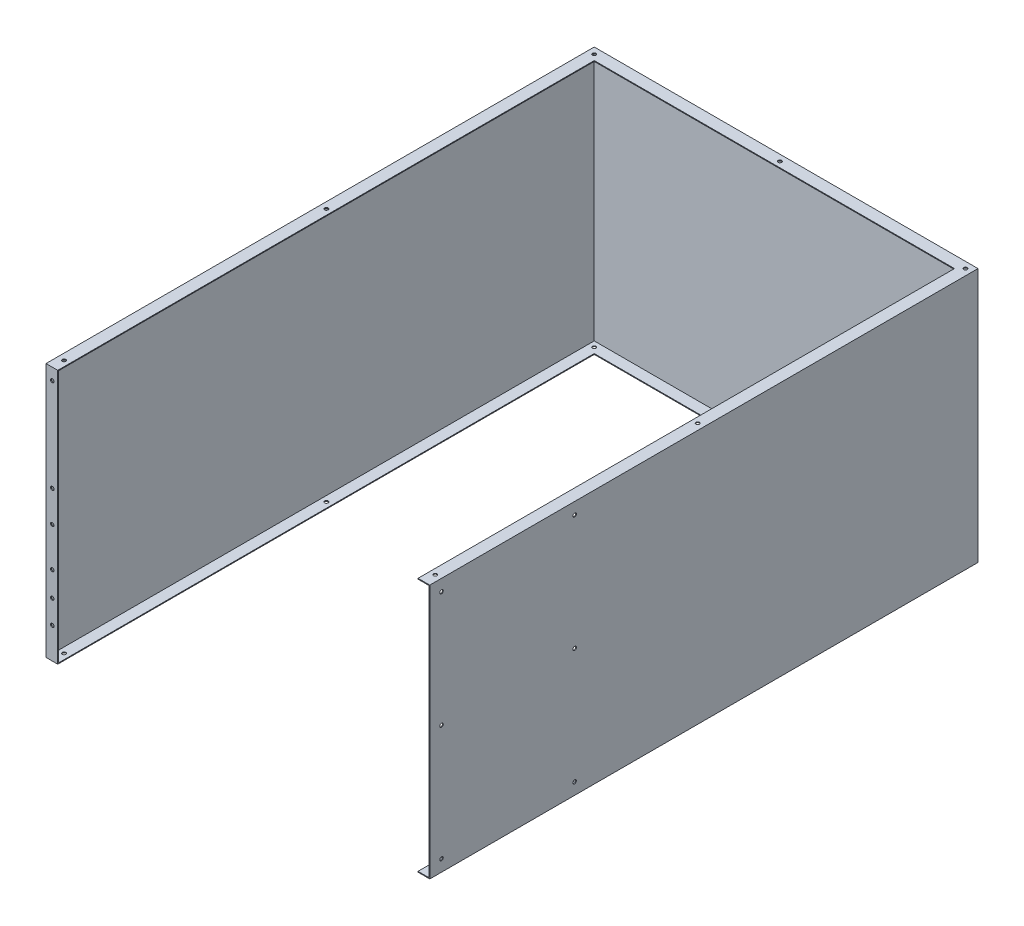
SolidWorks part; units mm, degrees
ref_plane "前视" through (0, 0, 0) normal (0, 0, 1) x (1, 0, 0)
ref_plane "上视" through (0, 0, 0) normal (0, 1, 0) x (1, 0, 0)
ref_plane "右视" through (0, 0, 0) normal (1, 0, 0) x (0, 0, -1)
sketch "草图1" plane through (0, 0, 0) normal (0, 1, 0) x (1, 0, 0)
  line L0 (0, 0) -> (0, 59.963) construction
  line L1 (0, 0) -> (65.7983, 0) construction
  line L2 (-490, 700) -> (490, 700)
  line L3 (490, 700) -> (490, -700)
  line L4 (-490, 700) -> (-490, -700)
  line L5 (-490, -700) -> (-488, -700)
  line L6 (-488, -700) -> (-488, 698)
  line L7 (490, -700) -> (488, -700)
  line L8 (488, -700) -> (488, 698)
  line L9 (488, 698) -> (-488, 698)
  dimension "D1" = 700
  dimension "D2" = 980
  dimension "D3" = 1400
  dimension "D4" = 490
  dimension "D5" = 1398
extrude "凸台-拉伸1" add sketch "草图1" along normal mid plane 650
sketch "草图2" plane through (0, 325, 0) normal (0, 1, 0) x (1, 0, 0)
  line L0 (-490, 700) -> (-490, -700)
  line L1 (-490, -700) -> (-460, -700)
  line L2 (-490, 700) -> (490, 700)
  line L3 (490, 700) -> (490, -700)
  line L4 (490, -700) -> (460, -700)
  line L5 (460, -700) -> (460, 670)
  line L6 (-460, -700) -> (-460, 670)
  line L7 (-460, 670) -> (460, 670)
  dimension "D1" = 30
  dimension "D2" = 30
  dimension "D3" = 30
extrude "凸台-拉伸2" add sketch "草图2" against normal blind 2
sketch "草图3" plane through (0, -325, 0) normal (0, -1, 0) x (1, 0, 0)
  line L0 (490, -700) -> (490, 700)
  line L1 (490, 700) -> (460, 700)
  line L2 (460, 700) -> (460, -670)
  line L3 (460, -670) -> (-460, -670)
  line L4 (-460, 700) -> (-460, -670) construction
  line L5 (-460, -670) -> (460, -670) construction
  line L6 (-460, -670) -> (-460, 700)
  line L7 (-460, 700) -> (-490, 700)
  line L8 (-490, 700) -> (-490, -700)
  line L9 (-490, -700) -> (490, -700)
extrude "凸台-拉伸3" add sketch "草图3" against normal blind 2
sketch "草图5" plane through (0, 0, 700) normal (0, 0, 1) x (1, 0, 0)
  line L0 (-490, 325) -> (-490, -325)
  line L1 (-490, -325) -> (-460, -325)
  line L2 (-460, -325) -> (-460, 325)
  line L3 (-460, 325) -> (-490, 325)
extrude "凸台-拉伸4" add sketch "草图5" against normal blind 2
ref_plane "基准面1" through (0, 150, 0) normal (0, 1, 0) x (-1, 0, 0)
sketch "草图6" plane through (0, 0, 698) normal (0, 0, -1) x (-1, 0, 0)
  line L0 (474, -323) -> (474, 491.326) construction
  line L1 (460, -323) -> (488, -323) construction
  line L2 (490, -325) -> (460, -325) construction
  line L3 (490, 325) -> (460, 325) construction
  circle A0 centre (474, -246) radius 4.5
  circle A1 centre (474, -186) radius 4.5
  circle A2 centre (474, 295) radius 4.5
  circle A3 centre (474, 57) radius 4.5
  circle A4 centre (474, -23) radius 4.5
  circle A5 centre (474, -123) radius 4.5
  dimension "D1" = 9
  dimension "D2" = 79
  dimension "D3" = 9
  dimension "D4" = 60
  dimension "D5" = 9
  dimension "D6" = 9
  dimension "D7" = 30
  dimension "D8" = 238
  dimension "D9" = 9
  dimension "D10" = 9
  dimension "D11" = 100
  dimension "D12" = 80
extrude "切除-拉伸1" cut sketch "草图6" against normal blind 10
sketch "草图7" plane through (0, 323, 0) normal (0, -1, 0) x (1, 0, 0)
  line L0 (-490, 0) -> (665.5888, 0) construction
  line L1 (-490, -700) -> (-490, 700) construction
  line L6 (-490, 700) -> (-460, 700) construction
  line L8 (0, -684) -> (0, -30.3843) construction
  line L9 (474, 700) -> (474, -684)
  line L10 (474, -684) -> (-474, -684)
  line L11 (-474, -684) -> (-474, 700)
  line L12 (474, 700) -> (474, -684) construction
  line L13 (474, -684) -> (-474, -684) construction
  line L14 (-474, -684) -> (-474, 700) construction
  circle A0 centre (-474, 670) radius 4.5
  circle A1 centre (-474, 0) radius 4.5
  circle A2 centre (-474, -684) radius 4.5
  circle A3 centre (474, -684) radius 4.5
  circle A4 centre (0, -684) radius 4.5
  circle A5 centre (474, 0) radius 4.5
  circle A6 centre (474, 670) radius 4.5
  dimension "D2" = 9
  dimension "D4" = 9
  dimension "D5" = 9
  dimension "D6" = 9
  dimension "D7" = 30
  dimension "D1" = 14
extrude "切除-拉伸2" cut sketch "草图7" against normal blind 345 and the other way blind 1140
sketch "草图8" plane through (490, 0, 0) normal (1, 0, 0) x (0, 0, -1)
  line L0 (-700, 0) -> (178.7458, 0) construction
  line L1 (-670, 295) -> (-330, 295) construction
  line L2 (-670, 295) -> (-670, -295) construction
  line L3 (-670, -295) -> (-330, -295) construction
  line L4 (-330, 295) -> (-330, -295) construction
  line L5 (-700, 325) -> (-700, -325) construction
  line L6 (-700, 325) -> (700, 325) construction
  circle A0 centre (-330, 295) radius 4.5
  circle A1 centre (-670, 295) radius 4.5
  circle A2 centre (-670, -295) radius 4.5
  circle A3 centre (-330, -295) radius 4.5
  circle A4 centre (-330, 0) radius 4.5
  circle A5 centre (-670, 0) radius 4.5
  dimension "D5" = 9
  dimension "D6" = 9
  dimension "D2" = 9
  dimension "D7" = 9
  dimension "D1" = 30
  dimension "D3" = 30
  dimension "D4" = 340
extrude "切除-拉伸3" cut sketch "草图8" against normal blind 10
